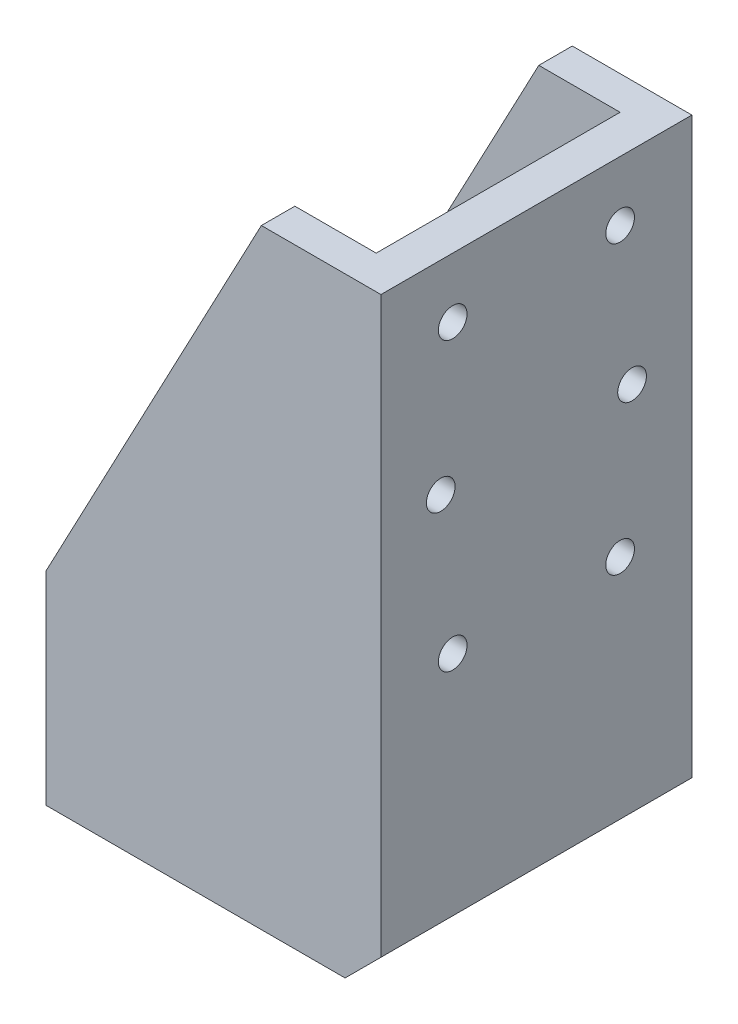
from build123d import *

# Parameters (mm, degrees)
EXTRUDE_1_DEPTH             = 130
SKETCH_2_W                  = 140
SKETCH_2_H                  = 5
CUT_EXTRUDE_1_DEPTH         = 323.645316098
SKETCH_3_W                  = 102
SKETCH_3_H                  = 170
CUT_EXTRUDE_2_DEPTH         = 124
CUT_EXTRUDE_3_DEPTH         = 323.645316098
HOLE_WIZARD_M14_1_D         = 12
HOLE_WIZARD_M14_1_DEPTH     = 34
HOLE_WIZARD_M14_1_TIP       = 3.605163714
HOLE_WIZARD_12_0_12_1_D     = 12
HOLE_WIZARD_12_0_12_1_DEPTH = 34
HOLE_WIZARD_12_0_12_1_TIP   = 3.605163714
CUT_EXTRUDE_4_REACH         = 302.299
SKETCH_12_R                 = 22.5


with BuildPart() as part:
    # 草图1 → 凸台-拉伸1 (new body)
    with BuildSketch(Plane.XY):
        Polygon((0, 0), (-140, 0), (-140, 90), (-50, 260), (0, 260), align=None)
    extrude(amount=EXTRUDE_1_DEPTH)

    # 草图2 → 切除-拉伸1 (cut, through all)
    with BuildSketch(Plane.XY.offset(130)):
        with Locations((-70, 2.5)):
            Rectangle(SKETCH_2_W, SKETCH_2_H)
    extrude(amount=-CUT_EXTRUDE_1_DEPTH, mode=Mode.SUBTRACT)

    # 草图3 → 切除-拉伸2 (cut)
    with BuildSketch(Plane(origin=(-140, 34.772640959, 0), x_dir=(0, 0, -1), z_dir=(1, 0, 0))):
        with Locations((-65, 140.227359041)):
            Rectangle(SKETCH_3_W, SKETCH_3_H)
    extrude(amount=CUT_EXTRUDE_2_DEPTH, mode=Mode.SUBTRACT)

    # 草图5 → 切除-拉伸3 (cut, through all)
    with BuildSketch(Plane.XY.offset(130)):
        Polygon((0, 5), (0, 20), (-15, 5), align=None)
    extrude(amount=-CUT_EXTRUDE_3_DEPTH, mode=Mode.SUBTRACT)

    # M14 螺纹孔1
    with Locations(Plane(origin=(0, 0, 0), x_dir=(0, 0, -1), z_dir=(1, 0, 0))):
        with Locations((-100, 235), (-30, 235), (-100, 115), (-30, 115)):
            Hole(HOLE_WIZARD_M14_1_D / 2, depth=HOLE_WIZARD_M14_1_DEPTH)
            with Locations((0, 0, -(HOLE_WIZARD_M14_1_DEPTH + HOLE_WIZARD_M14_1_TIP / 2))):  # 118° drill point
                Cone(0, HOLE_WIZARD_M14_1_D / 2, HOLE_WIZARD_M14_1_TIP, mode=Mode.SUBTRACT)

    # Ø12.0 (12) 直径孔1
    with Locations(Plane(origin=(0, 0, 0), x_dir=(0, 0, -1), z_dir=(1, 0, 0))):
        with Locations((-105, 175), (-25, 175)):
            Hole(HOLE_WIZARD_12_0_12_1_D / 2, depth=HOLE_WIZARD_12_0_12_1_DEPTH)
            with Locations((0, 0, -(HOLE_WIZARD_12_0_12_1_DEPTH + HOLE_WIZARD_12_0_12_1_TIP / 2))):  # 118° drill point
                Cone(0, HOLE_WIZARD_12_0_12_1_D / 2, HOLE_WIZARD_12_0_12_1_TIP, mode=Mode.SUBTRACT)

    # 草图12 → 切除-拉伸4 (cut, up to next)
    with BuildSketch(Plane(origin=(-90.854033512, 5, 0), x_dir=(-1, 0, 0), z_dir=(0, 1, 0)), mode=Mode.PRIVATE) as cut_extrude_4_sk1:
        with Locations(Location((-0.854033512, 63, 0), (0, 0, 90))):
            Circle(SKETCH_12_R)
    cut_extrude_4_tool1 = extrude(cut_extrude_4_sk1.sketch, amount=CUT_EXTRUDE_4_REACH, mode=Mode.PRIVATE) & part.part
    add(cut_extrude_4_tool1.solids().sort_by_distance((-90, 5, 63))[0], mode=Mode.SUBTRACT)


solid = part.part
